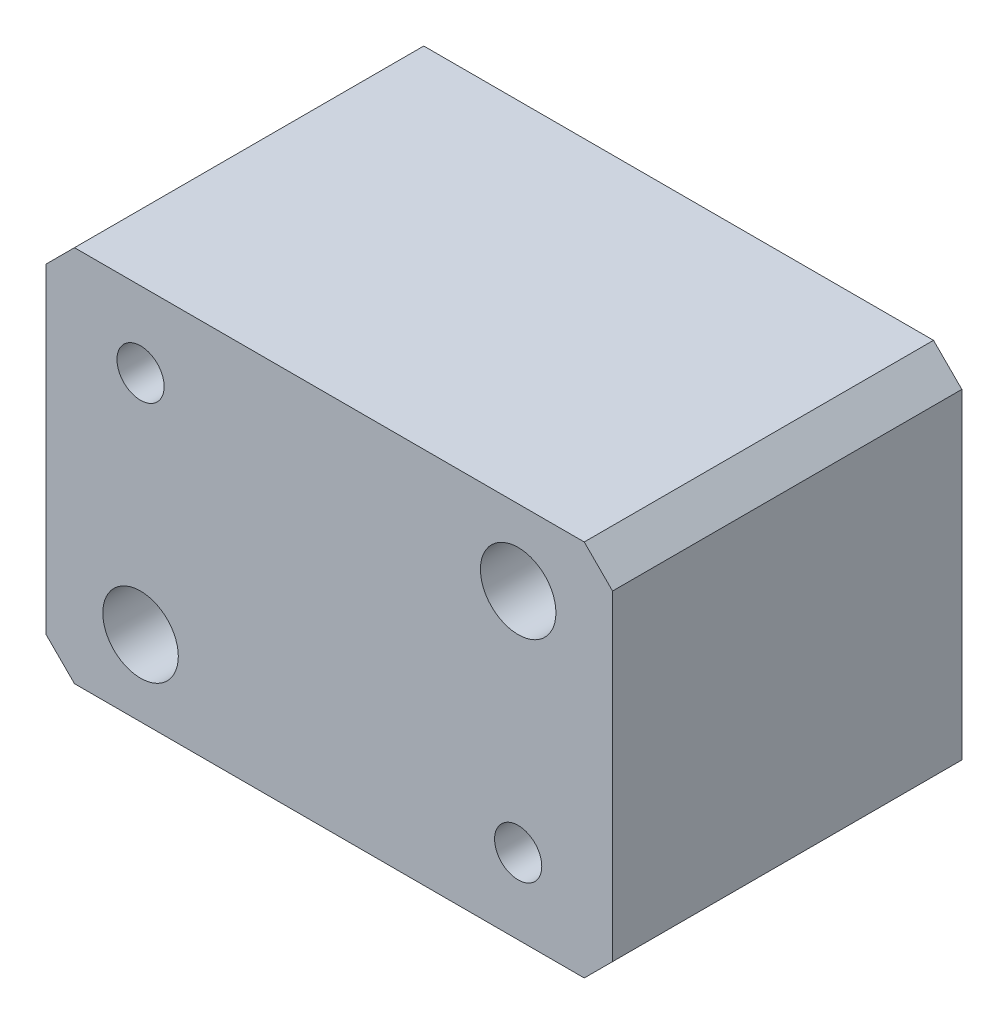
SolidWorks part; units mm, degrees
material "Q235-A"
ref_plane "Front Plane" through (0, 0, 0) normal (0, 0, 1) x (1, 0, 0)
ref_plane "Top Plane" through (0, 0, 0) normal (0, 1, 0) x (1, 0, 0)
ref_plane "Right Plane" through (0, 0, 0) normal (1, 0, 0) x (0, 0, -1)
sketch "Sketch1" plane through (0, 0, 0) normal (0, 0, 1) x (1, 0, 0)
  line L1 (-34.5021, 50.1923) -> (25.4979, 50.1923)
  line L2 (-34.5021, 50.1923) -> (-34.5021, 10.1923)
  line L3 (-34.5021, 10.1923) -> (25.4979, 10.1923)
  line L4 (25.4979, 50.1923) -> (25.4979, 10.1923)
  dimension "D1" = 60
  dimension "D2" = 40
extrude "Boss-Extrude1" add sketch "Sketch1" along normal blind 37
chamfer "Chamfer1" distance 3 angle 45 4 edges at (25.4979, 10.1923, 18.5) (25.4979, 50.1923, 18.5) (-34.5021, 10.1923, 18.5) (-34.5021, 50.1923, 18.5)
sketch "Sketch2" plane through (0, 0, 37) normal (0, 0, 1) x (1, 0, 0)
  line L0 (25.4979, 13.1923) -> (25.4979, 47.1923) construction
  line L1 (-24.5021, 42.1923) -> (15.4979, 42.1923)
  line L2 (-24.5021, 42.1923) -> (-24.5021, 18.1923)
  line L3 (-24.5021, 18.1923) -> (15.4979, 18.1923)
  line L4 (15.4979, 42.1923) -> (15.4979, 18.1923)
  line L5 (-31.5021, 10.1923) -> (22.4979, 10.1923) construction
  dimension "D1" = 40
  dimension "D2" = 24
  dimension "D3" = 10
  dimension "D4" = 8
sketch "Sketch3" plane through (0, 0, 0) normal (0, 0, -1) x (-1, 0, 0)
  line L4 (24.5021, 42.1923) -> (-15.4979, 42.1923)
  line L5 (-15.4979, 42.1923) -> (-15.4979, 18.1923)
  line L6 (-15.4979, 18.1923) -> (24.5021, 18.1923)
  line L7 (24.5021, 18.1923) -> (24.5021, 42.1923)
  line L8 (24.5021, 42.1923) -> (-15.4979, 42.1923)
  line L9 (-15.4979, 42.1923) -> (-15.4979, 18.1923)
  line L10 (-15.4979, 18.1923) -> (24.5021, 18.1923)
  line L11 (24.5021, 18.1923) -> (24.5021, 42.1923)
  dimension "D1" = 0
hole_wizard "M6 Tapped Hole1" positions "Sketch4" profile "Sketch5" tap size "M6" standard "GB"
sketch "Sketch4" plane through (0, 0, 37) normal (0, 0, 1) x (1, 0, 0)
  point P14 (-24.5021, 42.1923)
  point P17 (15.4979, 18.1923)
sketch "Sketch5" plane through (-24.5021, 42.1923, 37) normal (1, 0, 0) x (0, -1, 0)
  line L0 (0, 0) -> (0, 13.5022)
  line L1 (0, 13.5022) -> (2.5, 12)
  line L2 (2.5, 12) -> (2.5, 0)
  line L5 (2.5, 0) -> (0, 0)
  line L10 (0, 13.5022) -> (-2.5, 12) construction
  line L11 (0, -6.35) -> (0, 107.95) construction
  dimension "螺纹孔钻头直径" = 5
  dimension "螺纹孔钻头深度" = 12
  dimension "导头角度" = 118
cosmetic thread "Cosmetic thread 11" parameters "D1"=12, "D2"=6
cosmetic thread "Cosmetic thread 12" parameters "D1"=12, "D2"=6
hole_wizard "Hole1" positions "Sketch6" profile "Sketch7" legacy
sketch "Sketch6" plane through (0, 0, 37) normal (0, 0, 1) x (1, 0, 0)
  point P14 (15.4979, 42.1923)
  point P17 (-24.5021, 18.1923)
sketch "Sketch7" plane through (15.4979, 42.1923, 37) normal (1, 0, 0) x (0, -1, 0)
  line L0 (0, 0) -> (0, 10)
  line L1 (0, 10) -> (4, 10)
  line L2 (4, 10) -> (4, 0)
  line L3 (4, 0) -> (0, 0)
  line L4 (0, 110) -> (0, -10) construction
  dimension "直径" = 8
  dimension "深度" = 10
hole_wizard "Hole2" positions "Sketch8" profile "Sketch9" legacy
sketch "Sketch8" plane through (0, 0, 0) normal (0, 0, -1) x (-1, 0, 0)
  point P22 (24.5021, 42.1923)
  point P25 (-15.4979, 18.1923)
sketch "Sketch9" plane through (-24.5021, 42.1923, 0) normal (1, 0, 0) x (0, 1, 0)
  line L0 (0, 0) -> (0, 10)
  line L1 (0, 10) -> (4, 10)
  line L2 (4, 10) -> (4, 0)
  line L3 (4, 0) -> (0, 0)
  line L4 (0, 110) -> (0, -10) construction
  dimension "直径" = 8
  dimension "深度" = 10
hole_wizard "M6 Tapped Hole2" positions "Sketch10" profile "Sketch11" tap size "M6" standard "GB"
sketch "Sketch10" plane through (0, 0, 0) normal (0, 0, -1) x (-1, 0, 0)
  point P0 (-15.4979, 42.1923)
  point P3 (24.5021, 18.1923)
sketch "Sketch11" plane through (15.4979, 42.1923, 0) normal (1, 0, 0) x (0, 1, 0)
  line L0 (0, 0) -> (0, 13.5022)
  line L1 (0, 13.5022) -> (2.5, 12)
  line L2 (2.5, 12) -> (2.5, 0.525)
  line L3 (2.5, 0.525) -> (3.025, 0)
  line L5 (3.025, 0) -> (0, 0)
  line L6 (-2.5, 0.525) -> (-3.025, 0) construction
  line L10 (0, 13.5022) -> (-2.5, 12) construction
  line L11 (0, -6.35) -> (0, 107.95) construction
  dimension "螺纹孔钻头直径" = 5
  dimension "螺纹孔钻头深度" = 12
  dimension "近端锥形沉头孔直径" = 6.05
  dimension "近端锥形沉头孔角度" = 90
  dimension "导头角度" = 118
cosmetic thread "Cosmetic thread 9"
cosmetic thread "Cosmetic thread 10"
